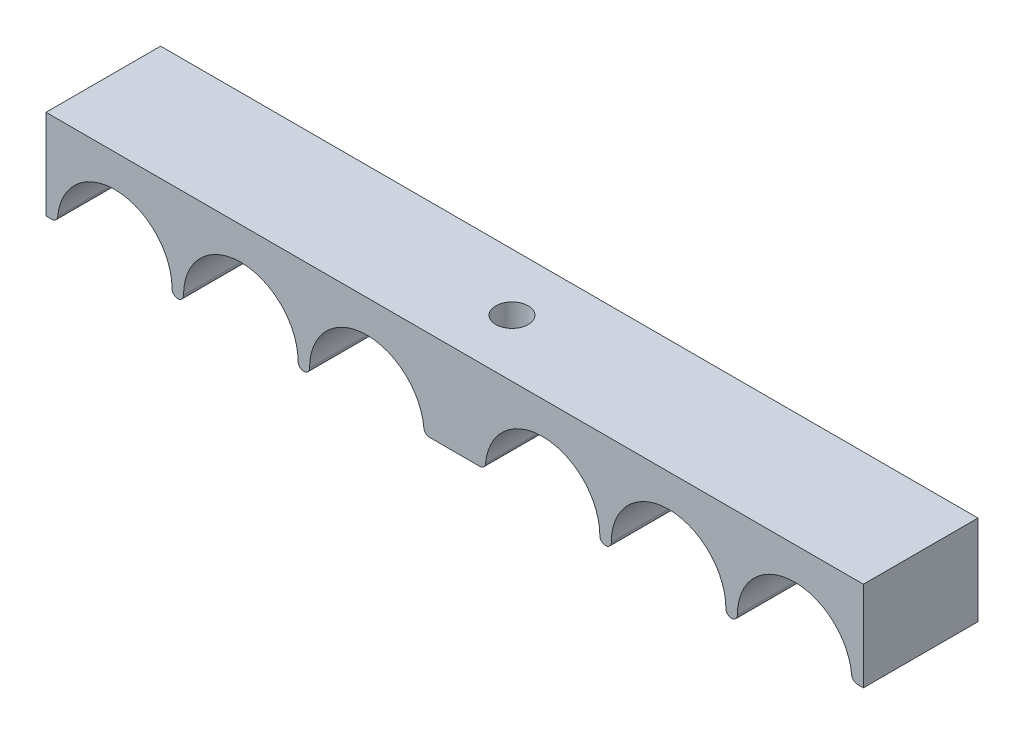
from build123d import *

# Parameters (mm, degrees)
BOSS_EXTRUDE1_DEPTH = 30
M10_TAPPED_HOLE1_D  = 8.5


with BuildPart() as part:
    # Sketch1 → Boss-Extrude1 (new body)
    with BuildSketch(Plane.XY):
        with BuildLine():
            Line((-107, 0), (-107, 23.5))
            Line((-107, 23.5), (107, 23.5))
            Line((107, 23.5), (107, 0))
            Line((107, 0), (105.431676725, 0))
            ThreePointArc((105.431676725, 0), (104.420376931, 0.392176581), (103.937887932, 1.363636364))
            ThreePointArc((103.937887932, 1.363636364), (88.317474901, 14.984463937), (74, 0))
            ThreePointArc((74, 0), (72.5, -1.5), (71, 0))
            ThreePointArc((71, 0), (56, 15), (41, 0))
            ThreePointArc((41, 0), (39.5, -1.5), (38, 0))
            ThreePointArc((38, 0), (23.682525099, 14.984463937), (8.062112068, 1.363636364))
            ThreePointArc((8.062112068, 1.363636364), (7.579623069, 0.392176581), (6.568323275, 0))
            Line((6.568323275, 0), (-6.568323275, 0))
            ThreePointArc((-6.568323275, 0), (-7.579623069, 0.392176581), (-8.062112068, 1.363636364))
            ThreePointArc((-8.062112068, 1.363636364), (-23.682525099, 14.984463937), (-38, 0))
            ThreePointArc((-38, 0), (-39.5, -1.5), (-41, 0))
            ThreePointArc((-41, 0), (-56, 15), (-71, 0))
            ThreePointArc((-71, 0), (-72.5, -1.5), (-74, 0))
            ThreePointArc((-74, 0), (-88.317474901, 14.984463937), (-103.937887932, 1.363636364))
            ThreePointArc((-103.937887932, 1.363636364), (-104.420376931, 0.392176581), (-105.431676725, 0))
            Line((-105.431676725, 0), (-107, 0))
        make_face()
    extrude(amount=BOSS_EXTRUDE1_DEPTH)

    # M10 Tapped Hole1 (through all)
    with Locations(Plane(origin=(0, 23.5, 0), x_dir=(-1, 0, 0), z_dir=(0, 1, 0))):
        with Locations((0, 15)):
            Hole(M10_TAPPED_HOLE1_D / 2)


solid = part.part
